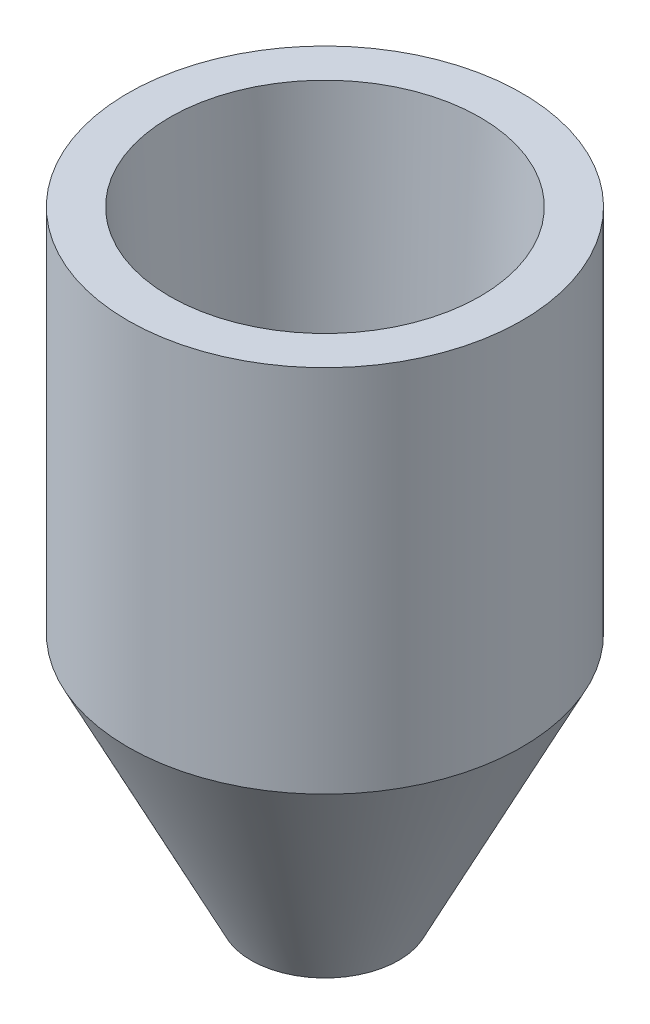
SolidWorks part; units mm, degrees
material "CuCrZr"
ref_plane "前视基准面" through (0, 0, 0) normal (0, 0, 1) x (1, 0, 0)
ref_plane "上视基准面" through (0, 0, 0) normal (0, 1, 0) x (1, 0, 0)
ref_plane "右视基准面" through (0, 0, 0) normal (1, 0, 0) x (0, 0, -1)
sketch "草图1" plane through (0, 0, 0) normal (0, 1, 0) x (1, 0, 0)
  circle A0 centre (0, 0) radius 8
  dimension "D1" = 16
extrude "凸台-拉伸1" add sketch "草图1" along normal blind 25
sketch "草图2" plane through (0, 25, 0) normal (0, 1, 0) x (1, 0, 0)
  circle A0 centre (0, 0) radius 6.3
  dimension "D1" = 12.6
chamfer "倒角2" distance 5 distance2 10 1 edges at (0, 0, 8)
sketch "草图3" plane through (0, 0, 0) normal (1, 0, 0) x (0, 0, -1)
  line L0 (0, 25) -> (0, 0) construction
  line L1 (6.3, 25) -> (-6.3, 25) construction
  line L2 (0, 25) -> (0.5, 25) construction
  line L3 (0.5, 25) -> (0, 15) construction
  line L4 (6.3, 25) -> (5.75, 14)
  line L5 (8, 25) -> (-8, 25) construction
  line L6 (5.75, 14) -> (0, 14)
  line L7 (6.3, 25) -> (0, 25)
  line L8 (0, 25) -> (0, 14)
  dimension "D1" = 0.5
  dimension "D2" = 10
  dimension "D3" = 12.6
  dimension "D4" = 11
revolve "切除-旋转1" cut sketch "草图3" angle 360 about L0
